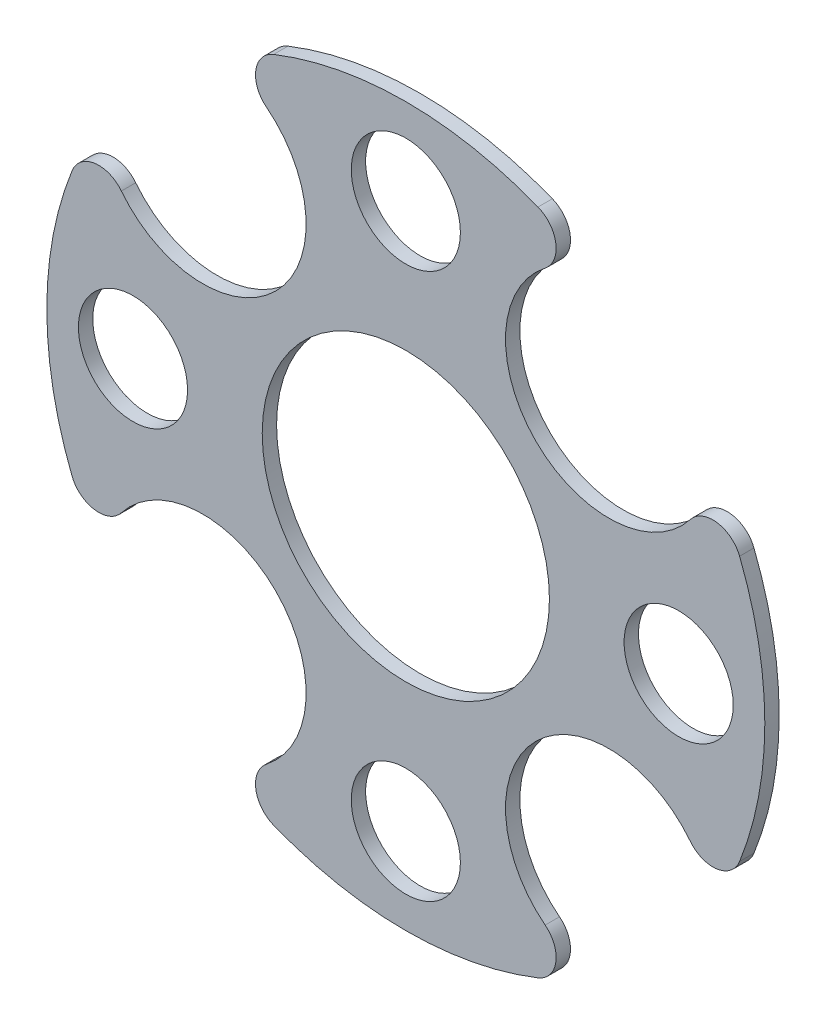
from build123d import *

# Parameters (mm, degrees)
SKETCH1_R           = 5
SKETCH1_R_2         = 1.9
BOSS_EXTRUDE1_DEPTH = 0.5


with BuildPart() as part:
    # Sketch1 → Boss-Extrude1 (new body)
    with BuildSketch(Plane.XY):
        with BuildLine():
            ThreePointArc((-11.621881793, 4.602375864), (-12.5, 0), (-11.621881793, -4.602375864))
            ThreePointArc((-11.621881793, -4.602375864), (-10.835386311, -5.223871597), (-9.904943546, -4.850899277))
            ThreePointArc((-9.904943546, -4.850899277), (-4.5254834, -4.5254834), (-4.850899277, -9.904943546))
            ThreePointArc((-4.850899277, -9.904943546), (-5.223871597, -10.835386311), (-4.602375864, -11.621881793))
            ThreePointArc((-4.602375864, -11.621881793), (0, -12.5), (4.602375864, -11.621881793))
            ThreePointArc((4.602375864, -11.621881793), (5.223871597, -10.835386311), (4.850899277, -9.904943546))
            ThreePointArc((4.850899277, -9.904943546), (4.5254834, -4.5254834), (9.904943546, -4.850899277))
            ThreePointArc((9.904943546, -4.850899277), (10.835386311, -5.223871597), (11.621881793, -4.602375864))
            ThreePointArc((11.621881793, -4.602375864), (12.5, 0), (11.621881793, 4.602375864))
            ThreePointArc((11.621881793, 4.602375864), (10.835386311, 5.223871597), (9.904943546, 4.850899277))
            ThreePointArc((9.904943546, 4.850899277), (4.5254834, 4.5254834), (4.850899277, 9.904943546))
            ThreePointArc((4.850899277, 9.904943546), (5.223871597, 10.835386311), (4.602375864, 11.621881793))
            ThreePointArc((4.602375864, 11.621881793), (0, 12.5), (-4.602375864, 11.621881793))
            ThreePointArc((-4.602375864, 11.621881793), (-5.223871597, 10.835386311), (-4.850899277, 9.904943546))
            ThreePointArc((-4.850899277, 9.904943546), (-4.5254834, 4.5254834), (-9.904943546, 4.850899277))
            ThreePointArc((-9.904943546, 4.850899277), (-10.835386311, 5.223871597), (-11.621881793, 4.602375864))
        make_face()
        Circle(SKETCH1_R, mode=Mode.SUBTRACT)
        with Locations((0, 9.5)):
            Circle(SKETCH1_R_2, mode=Mode.SUBTRACT)
        with Locations((9.5, 0)):
            Circle(SKETCH1_R_2, mode=Mode.SUBTRACT)
        with Locations((0, -9.5)):
            Circle(SKETCH1_R_2, mode=Mode.SUBTRACT)
        with Locations((-9.5, 0)):
            Circle(SKETCH1_R_2, mode=Mode.SUBTRACT)
    extrude(amount=BOSS_EXTRUDE1_DEPTH)


solid = part.part
